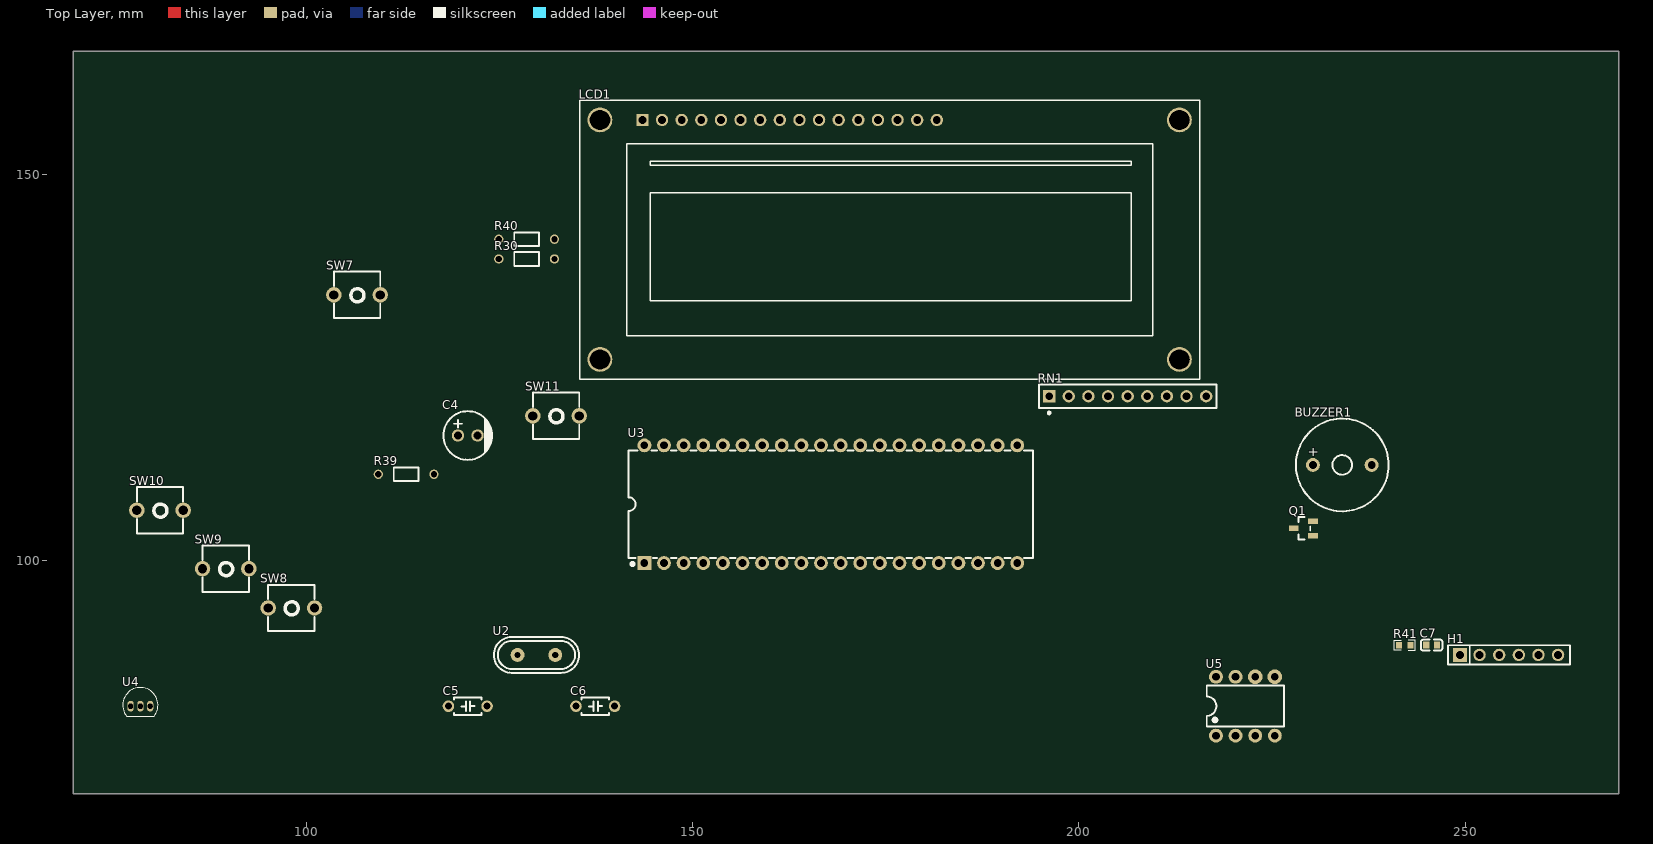
[diagram p0: Top Layer view]
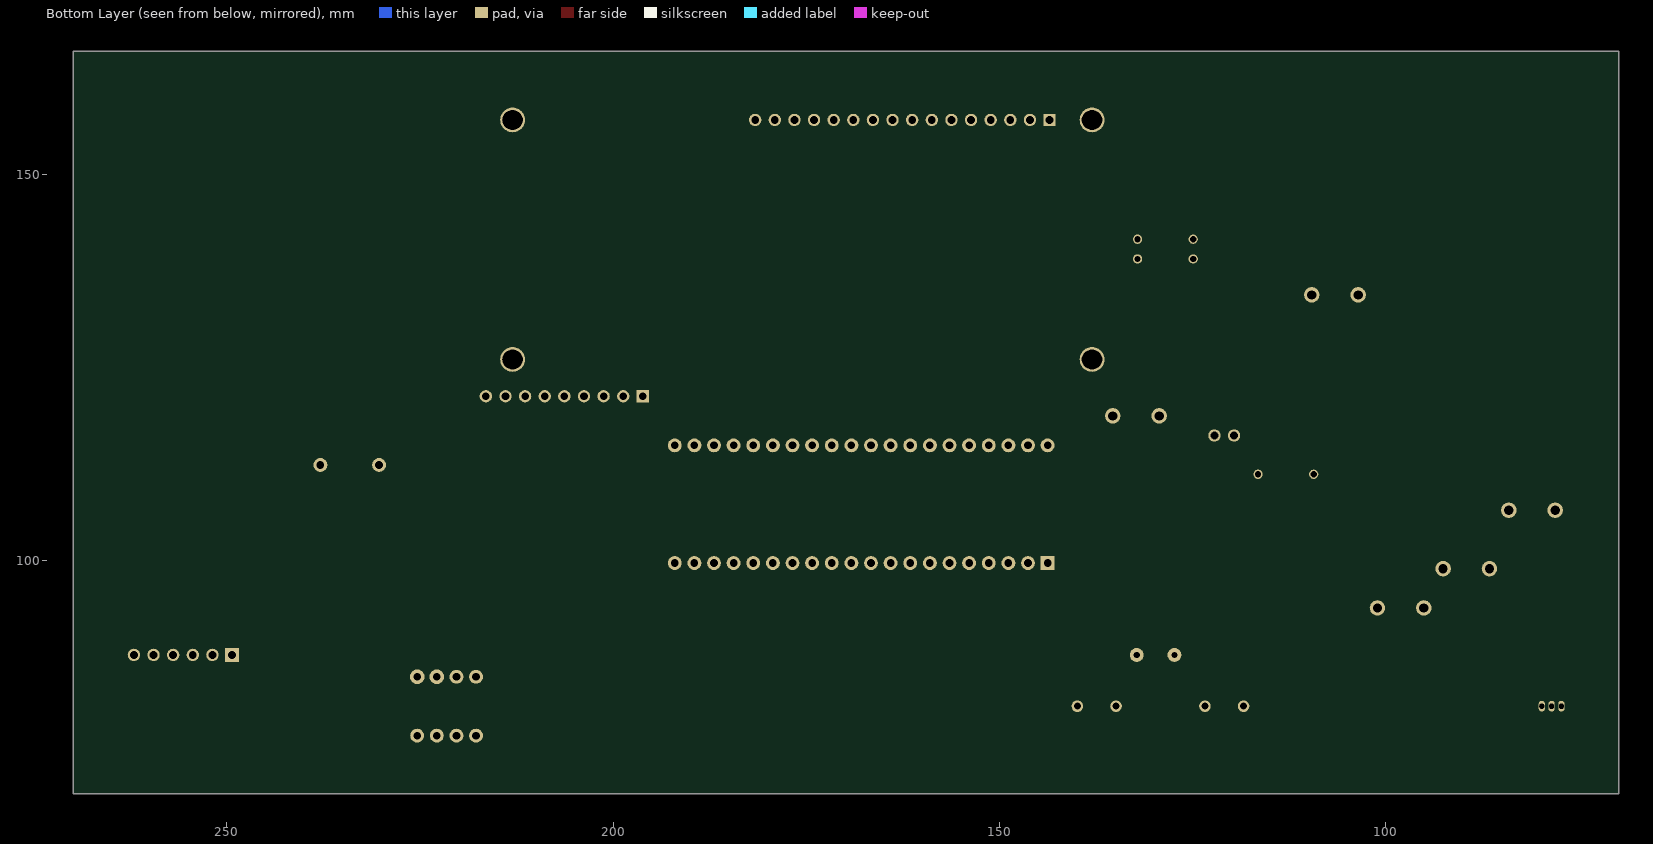
[diagram p1: Bottom Layer view, seen from below]
# Altium PCB MISC49895.pcbdoc
Units mm, origin at the board's own origin, x right, y up, seen from the top; angles counter-clockwise.
Board outline 200.06 x 96.14 mm, 2 copper layers (Top Layer, Bottom Layer), stack 1.58 mm thick; 22 components, 27 nets, 119 pads, 0 vias.

## Layer stack, top to bottom
Top Solder Mask Layer: solder mask 0.01, Dk 3.3
Top Layer: signal copper 0.035
Dielectric1: surface 1.51, FR4, Dk 4.5
Bottom Layer: signal copper 0.035
Bottom Solder Mask Layer: solder mask 0.01, Dk 3.3

## Board outline
269.911,69.85 69.85,69.85 69.85,165.986 269.911,165.986

## Design rules (kind name [scope] priority, off if disabled: settings)
BoardOutlineClearance copperThickness2oz_1 [All] p2 off: genericclearance=0.203 ignorepadtopadclearanceinfootprint=FALSE except(0: Arc-SplitContinuation Track-SplitContinuation SMDPad-SplitContinuation THPad-SplitContinuation Via-SplitContinuation Fill-SplitContinuation Region-SplitContinuation Poly-SplitContinuation Text-SplitContinuation Hole-SplitContinuation; 0.152: Arc-CutoutEdge Track-CutoutEdge SMDPad-CutoutEdge THPad-CutoutEdge Via-CutoutEdge Text-CutoutEdge; 0.175: Hole-OutlineEdge Hole-CutoutEdge; 0.254: Poly-OutlineEdge Poly-CutoutEdge; 0.3: Arc-OutlineEdge Track-OutlineEdge SMDPad-OutlineEdge THPad-OutlineEdge Via-OutlineEdge Fill-OutlineEdge Region-OutlineEdge Text-OutlineEdge Fill-CutoutEdge Region-CutoutEdge)
BoardOutlineClearance Plane_innerPlane_1 [All] p4 off: genericclearance=0.102 ignorepadtopadclearanceinfootprint=FALSE except(0: Arc-SplitContinuation Track-SplitContinuation SMDPad-SplitContinuation THPad-SplitContinuation Via-SplitContinuation Fill-SplitContinuation Region-SplitContinuation Poly-SplitContinuation Text-SplitContinuation Hole-SplitContinuation; 0.152: Arc-CutoutEdge Track-CutoutEdge SMDPad-CutoutEdge THPad-CutoutEdge Via-CutoutEdge Text-CutoutEdge; 0.175: Hole-OutlineEdge Hole-CutoutEdge; 0.254: Poly-OutlineEdge Poly-CutoutEdge; 0.3: Arc-OutlineEdge Track-OutlineEdge SMDPad-OutlineEdge THPad-OutlineEdge Via-OutlineEdge Fill-OutlineEdge Region-OutlineEdge Text-OutlineEdge Fill-CutoutEdge Region-CutoutEdge)
BoardOutlineClearance Copper_copperRegion_1 [All] p6 off: genericclearance=0.102 ignorepadtopadclearanceinfootprint=FALSE except(0: Arc-SplitContinuation Track-SplitContinuation SMDPad-SplitContinuation THPad-SplitContinuation Via-SplitContinuation Fill-SplitContinuation Region-SplitContinuation Poly-SplitContinuation Text-SplitContinuation Hole-SplitContinuation; 0.152: Arc-CutoutEdge Track-CutoutEdge SMDPad-CutoutEdge THPad-CutoutEdge Via-CutoutEdge Text-CutoutEdge; 0.175: Hole-OutlineEdge Hole-CutoutEdge; 0.254: Poly-OutlineEdge Poly-CutoutEdge; 0.3: Arc-OutlineEdge Track-OutlineEdge SMDPad-OutlineEdge THPad-OutlineEdge Via-OutlineEdge Fill-OutlineEdge Region-OutlineEdge Text-OutlineEdge Fill-CutoutEdge Region-CutoutEdge)
BoardOutlineClearance copperThickness1oz_1 [All] p8: genericclearance=0.102 ignorepadtopadclearanceinfootprint=FALSE except(0: Arc-SplitContinuation Track-SplitContinuation SMDPad-SplitContinuation THPad-SplitContinuation Via-SplitContinuation Fill-SplitContinuation Region-SplitContinuation Poly-SplitContinuation Text-SplitContinuation Hole-SplitContinuation; 0.152: Arc-CutoutEdge Track-CutoutEdge SMDPad-CutoutEdge THPad-CutoutEdge Via-CutoutEdge Text-CutoutEdge; 0.175: Hole-OutlineEdge Hole-CutoutEdge; 0.254: Poly-OutlineEdge Poly-CutoutEdge; 0.3: Arc-OutlineEdge Track-OutlineEdge SMDPad-OutlineEdge THPad-OutlineEdge Via-OutlineEdge Fill-OutlineEdge Region-OutlineEdge Text-OutlineEdge Fill-CutoutEdge Region-CutoutEdge)
Clearance copperThickness2oz [All] p1 off: gap=0.203 ignorepadtopadclearanceinfootprint=FALSE except(0.152: SMDPad-Track SMDPad-SMDPad THPad-Track SMDPad-THPad THPad-THPad Track-Via SMDPad-Via THPad-Via Via-Via Fill-SMDPad Region-SMDPad Fill-THPad Region-THPad Fill-Via Region-Via Fill-Fill Fill-Region Region-Region Arc-Track Arc-SMDPad Arc-THPad Arc-Via Fill-Arc Region-Arc Arc-Arc Text-Track SMDPad-Text Text-THPad Text-Via Fill-Text Region-Text Arc-Text Text-Text; 0.175: Hole-Track Hole-SMDPad Hole-THPad Hole-Via Fill-Hole Region-Hole Hole-Arc Hole-Text; 0.254: Poly-Track Poly-SMDPad Poly-THPad Poly-Via Poly-Fill Poly-Region Poly-Poly Poly-Arc Poly-Text Poly-Hole; 0.3: Fill-Track Region-Track)
Clearance Plane_innerPlane [All] p3 off: gap=0.102 ignorepadtopadclearanceinfootprint=FALSE except(0.152: SMDPad-Track SMDPad-SMDPad THPad-Track SMDPad-THPad THPad-THPad Track-Via SMDPad-Via THPad-Via Via-Via Fill-SMDPad Region-SMDPad Fill-THPad Region-THPad Fill-Via Region-Via Fill-Fill Fill-Region Region-Region Arc-Track Arc-SMDPad Arc-THPad Arc-Via Fill-Arc Region-Arc Arc-Arc Text-Track SMDPad-Text Text-THPad Text-Via Fill-Text Region-Text Arc-Text Text-Text; 0.175: Hole-Track Hole-SMDPad Hole-THPad Hole-Via Fill-Hole Region-Hole Hole-Arc Hole-Text; 0.254: Poly-Track Poly-SMDPad Poly-THPad Poly-Via Poly-Fill Poly-Region Poly-Poly Poly-Arc Poly-Text Poly-Hole; 0.3: Fill-Track Region-Track)
Clearance Copper_copperRegion [All] p5 off: gap=0.102 ignorepadtopadclearanceinfootprint=FALSE except(0.152: SMDPad-Track SMDPad-SMDPad THPad-Track SMDPad-THPad THPad-THPad Track-Via SMDPad-Via THPad-Via Via-Via Fill-SMDPad Region-SMDPad Fill-THPad Region-THPad Fill-Via Region-Via Fill-Fill Fill-Region Region-Region Arc-Track Arc-SMDPad Arc-THPad Arc-Via Fill-Arc Region-Arc Arc-Arc Text-Track SMDPad-Text Text-THPad Text-Via Fill-Text Region-Text Arc-Text Text-Text; 0.175: Hole-Track Hole-SMDPad Hole-THPad Hole-Via Fill-Hole Region-Hole Hole-Arc Hole-Text; 0.254: Poly-Track Poly-SMDPad Poly-THPad Poly-Via Poly-Fill Poly-Region Poly-Poly Poly-Arc Poly-Text Poly-Hole; 0.3: Fill-Track Region-Track)
Clearance copperThickness1oz [All] p7: gap=0.102 ignorepadtopadclearanceinfootprint=FALSE except(0.152: SMDPad-Track SMDPad-SMDPad THPad-Track SMDPad-THPad THPad-THPad Track-Via SMDPad-Via THPad-Via Via-Via Fill-SMDPad Region-SMDPad Fill-THPad Region-THPad Fill-Via Region-Via Fill-Fill Fill-Region Region-Region Arc-Track Arc-SMDPad Arc-THPad Arc-Via Fill-Arc Region-Arc Arc-Arc Text-Track SMDPad-Text Text-THPad Text-Via Fill-Text Region-Text Arc-Text Text-Text; 0.175: Hole-Track Hole-SMDPad Hole-THPad Hole-Via Fill-Hole Region-Hole Hole-Arc Hole-Text; 0.254: Poly-Track Poly-SMDPad Poly-THPad Poly-Via Poly-Fill Poly-Region Poly-Poly Poly-Arc Poly-Text Poly-Hole; 0.3: Fill-Track Region-Track)
DiffPairsRouting differentialPair [All] p1: maxlimit=0.152 minlimit=0.152 mostfreqgap=0.152 toplayer_minwidth=0.127 toplayer_prefwidth=0.254 toplayer_maxwidth=2.54 toplayer_mingap=0.152 toplayer_prefgap=0.152 toplayer_maxgap=0.152 bottomlayer_minwidth=0.127 bottomlayer_prefwidth=0.254 bottomlayer_maxwidth=2.54 bottomlayer_mingap=0.152 bottomlayer_prefgap=0.152 bottomlayer_maxgap=0.152 maxuncoupledlength=0.254
HoleToHoleClearance otherClearance [All] p1: gap=0.3 allowstackedmicrovias=TRUE
Length netLength [All] p1: minlimit=0 maxlimit=0
PasteMaskExpansion pasteMaskExpansion [All] p1: expansion=0
PlaneConnect innerPlane [All] p1: planeconnectstyle=Relief reliefexpansion=0.508 reliefentries=4 reliefconductorwidth=0.254 reliefairgap=0.254
PolygonConnect copperRegion [All] p1: connectstyle=Relief reliefconductorwidth=0.254 reliefentries=4 polygonreliefangle="90 Angle" airgapwidth=0.254 via.connectstyle=Relief via.reliefconductorwidth=0.254 via.reliefentries=4 via.polygonreliefangle="90 Angle" via.airgapwidth=0.254
RoutingVias viaSize [All] p1: holewidth=0.305 width=0.61 viastyle="Through Hole" minholewidth=0.3 minwidth=0.5 maxholewidth=6.3 maxwidth=10
SolderMaskExpansion solderMaskExpansion [IsVia] p1: expansion=-25.4 istentingtop=TRUE
SolderMaskExpansion solderMaskExpansion [All] p2: expansion=0.051 istentingtop=FALSE
Width copperThickness2oz_2 [All] p1 off: maxlimit=2.54 minlimit=0.203 preferedwidth=0.254
Width copperThickness1oz_2 [All] p2: maxlimit=2.54 minlimit=0.127 preferedwidth=0.254

## Components (designator, comment, footprint, x,y, rotation, side; value= is the part's Value field where it differs from the comment)
BUZZER1 "buzzer-12X9" BUZ-TH_BD12.0-P7.60-D0.6-FD 234.111,112.425 r0 top
C4 "10uF" CAP-TH_BD6.3-P2.50-D1.0-FD 120.925,116.235 r0 top
C5 "30pF" CAP-TH_L3.6-W2.3-P5.00-D0.5 120.925,81.199 r0 top
C6 "30pF" CAP-TH_L3.6-W2.3-P5.00-D0.5 137.435,81.199 r0 top
C7 "22pF" C0603 245.677,89.108 r0 top
H1 "" HDR-TH_6P-P2.54-V-F 255.691,87.838 r0 top
LCD1 "LMB162ADC" LCD1602 175.535,141.576 r0 top
Q1 "" S8550P_SOT 229.031,104.211 r0 top
R30 "1kΩ" Res_1/8W 128.545,139.024 r0 top
R39 "10kΩ" Res_1/8W 112.95,111.155 r0 top
R40 "10kΩ" Res_1/8W 128.545,141.576 r0 top
R41 "51K" R0603 242.199,89.108 r0 top
RN1 "-" RES-ARRAY-TH_9P-P2.54-D1.0 206.331,121.315 r0 top
SW7 "Tact switch, 6*6*5 plastic head, 260G, travel 0.25mm, through-hole, middle 2 pins" KEY-TH_2P-L6.0-W6.0-P5.00 106.6,134.433 r0 top
SW8 "Tact switch, 6*6*5 plastic head, 260G, travel 0.25mm, through-hole, middle 2 pins" KEY-TH_2P-L6.0-W6.0-P5.00 98.1,93.916 r0 top
SW9 "Tact switch, 6*6*5 plastic head, 260G, travel 0.25mm, through-hole, middle 2 pins" KEY-TH_2P-L6.0-W6.0-P5.00 89.6,98.996 r0 top
SW10 "Tact switch, 6*6*5 plastic head, 260G, travel 0.25mm, through-hole, middle 2 pins" KEY-TH_2P-L6.0-W6.0-P5.00 81.1,106.565 r0 top
SW11 "Tact switch, 6*6*5 plastic head, 260G, travel 0.25mm, through-hole, middle 2 pins" KEY-TH_2P-L6.0-W6.0-P5.00 132.355,118.775 r0 top
U2 "12MHz" HC-49US_L11.0-W4.6-P4.88 129.815,87.838 r0 top
U3 "STC89C516RD+40I-PDIP40" DIP-40_L52.3-W13.9-P2.54-LS15.2-BL 167.915,107.345 r0 top
U4 "DS18B20" TO-92-3_L4.6-W3.6-P1.27-L-1 78.56,81.199 r0 top
U5 "ADC0832BCN" PDIP-8_L9.6-W6.4-P2.54-LS7.6-BL 221.571,81.199 r0 top

## Footprints (in the part's own frame and the unit in brackets; to place one, negate y for a bottom-side part, rotate by r counter-clockwise, add the part's x,y. Pads: shape width x height; smd on the part's side, far side on the other; paste and mask are expansions set on the pad)
BUZ-TH_BD12.0-P7.60-D0.6-FD [mm]
  round 1.8 hole 1: 1(-3.8,0) 2(3.8,0)
  silkscreen extent -6,-6 6,6
C0603 [mm]
  rect 0.8x0.9 smd: 1(-0.7,0) 2(0.7,0)
  silkscreen extent -1.39,-0.71 1.39,0.71
CAP-TH_BD6.3-P2.50-D1.0-FD [mm]
  round 1.6 hole 1: 1(-1.27,0) 2(1.27,0)
  silkscreen extent -3.15,-3.15 3.17,3.15
CAP-TH_L3.6-W2.3-P5.00-D0.5 [mm]
  round 1.5 hole 0.9: 1(-2.5,0) 2(2.5,0)
  silkscreen extent -1.8,-1.15 1.8,1.15
DIP-40_L52.3-W13.9-P2.54-LS15.2-BL [mm]
  rect 1.8x1.8 hole 1: 1(-24.13,-7.62)
  round 1.8 hole 1: 2(-21.59,-7.62) 3(-19.05,-7.62) 4(-16.51,-7.62) 5(-13.97,-7.62) 6(-11.43,-7.62) 7(-8.89,-7.62) 8(-6.35,-7.62) 9(-3.81,-7.62) 10(-1.27,-7.62) 11(1.27,-7.62) 12(3.81,-7.62) 13(6.35,-7.62) 14(8.89,-7.62) 15(11.43,-7.62) 16(13.97,-7.62) 17(16.51,-7.62) 18(19.05,-7.62) 19(21.59,-7.62) 20(24.13,-7.62) 21(24.13,7.62) 22(21.59,7.62) 23(19.05,7.62) 24(16.51,7.62) 25(13.97,7.62) 26(11.43,7.62) 27(8.89,7.62) 28(6.35,7.62) 29(3.81,7.62) 30(1.27,7.62) 31(-1.27,7.62) 32(-3.81,7.62) 33(-6.35,7.62) 34(-8.89,7.62) 35(-11.43,7.62) 36(-13.97,7.62) 37(-16.51,7.62) 38(-19.05,7.62) 39(-21.59,7.62) 40(-24.13,7.62)
  silkscreen extent -26.16,-7.95 26.16,6.93
HC-49US_L11.0-W4.6-P4.88 [mm]
  round 1.8 hole 0.8: 1(-2.44,0) 2(2.44,0)
  silkscreen extent -5.51,-2.32 5.51,2.32
HDR-TH_6P-P2.54-V-F [mm]
  rect 1.8x1.8 hole 1.02: 1(-6.35,0)
  round 1.6 hole 1.02: 2(-3.81,0) 3(-1.27,0) 4(1.27,0) 5(3.81,0) 6(6.35,0)
  silkscreen extent -7.87,-1.25 7.87,1.25
KEY-TH_2P-L6.0-W6.0-P5.00 [mm]
  round 2 hole 1.2: 1(-3,0) 2(3,0)
  silkscreen extent -3,-3 3,3
LCD1602 [mm]
  round 3.2 hole 2.5 slot 2.625 at 0 deg: 0(-37.5,-15.5) 0(-37.5,15.5) 0(37.5,-15.5) 0(37.5,15.5)
  rect 1.6x1.6 hole 1: 1(-32,15.5)
  round 1.6 hole 1: 2(-29.46,15.5) 3(-26.92,15.5) 4(-24.38,15.5) 5(-21.84,15.5) 6(-19.3,15.5) 7(-16.76,15.5) 8(-14.22,15.5) 9(-11.68,15.5) 10(-9.14,15.5) 11(-6.6,15.5) 12(-4.06,15.5) 13(-1.52,15.5) 14(1.02,15.5) 15(3.56,15.5) 16(6.1,15.5)
  silkscreen extent -40.13,-18.03 40.13,18.03
PDIP-8_L9.6-W6.4-P2.54-LS7.6-BL [mm]
  round 1.8 hole 1: 1(-3.81,-3.81) 2(-1.27,-3.81) 3(1.27,-3.81) 4(3.81,-3.81) 7(-1.27,3.81) 8(-3.81,3.81)
  round 1.905 hole 1: 5(3.81,3.81) 6(1.27,3.81)
  silkscreen extent -5,-2.64 5,2.67
R0603 [mm]
  rect 0.806x0.864 smd paste-100 mask+0.051: 1(-0.753,0) 2(0.753,0)
  silkscreen extent -1.39,-0.66 1.39,0.66
RES-ARRAY-TH_9P-P2.54-D1.0 [mm]
  rect 1.6x1.6 hole 1: 1(-10.16,0)
  round 1.6 hole 1: 2(-7.62,0) 3(-5.08,0) 4(-2.54,0) 5(0,0) 6(2.54,0) 7(5.08,0) 8(7.62,0) 9(10.16,0)
  silkscreen extent -11.5,-2.31 11.5,1.5
Res_1/8W [mil]
  round 47.2 hole 31.5 paste+0 mask+2: 1(-141.7,2.48) 2(141.7,2.48)
  silkscreen extent -63,-33 63,38
S8550P_SOT [mm]
  rect 1.25x0.701 smd paste+0 mask+0.051: 1(1.291,-0.95) 2(1.291,0.95) 3(-1.208,0)
  silkscreen extent -0.61,-1.46 0.94,1.46
TO-92-3_L4.6-W3.6-P1.27-L-1 [mm]
  oval 0.8x1.4 hole 0.6 slot 0.682 at 90 deg paste+0 mask+0.05: 1(-1.27,0) 2(0,0) 3(1.27,0)
  silkscreen extent -2.28,-1.28 2.28,2.41

## Nets (pads, with @x,y where several pads share a name; then routed paths per layer and width w, separated by ;. In a path a pad name is that pad's centre, name@x,y a point inside that pad or via, vN(x,y) a via of type N, cw(c..) or ccw(c..) an arc to the next point about the centre after c; other vN are vias at no path point)
$1N1586: LCD1.14 RN1.9 U3.32
$1N1590: LCD1.7 RN1.2 U3.39
$1N1591: LCD1.8 RN1.3 U3.38
$1N1592: LCD1.9 RN1.4 U3.37
$1N1593: LCD1.10 RN1.5 U3.36
$1N1594: LCD1.11 RN1.6 U3.35
$1N1595: LCD1.12 RN1.7 U3.34
$1N1596: LCD1.13 RN1.8 U3.33
$1N1605: LCD1.3 R30.2 R40.1
$1N1611: C5.2 U2.1 U3.18
$1N1612: C6.2 U2.2 U3.19
$1N1662: C4.2 R39.2 SW11.2 U3.9
$1N19376: SW7.2 U3.8
$1N19435: SW10.2 U3.10
$1N19444: SW9.2 U3.11
$1N19454: SW8.2 U3.12
$1N19651: U3.17 U4.2
$1N19796: U3.23 U5.1
$1N19863: U3.24 U5.7
$1N19872: U3.25 U5.5 U5.6
$1N19973: C7.2 H1.1 R41.2 U5.2
$1N20248: BUZZER1.2 Q1.2
EN: LCD1.6
GND: C5.1 C6.1 C7.1 H1.2 LCD1.1 LCD1.16 Q1.3 R30.1 R39.1 R41.1 SW7.1 SW8.1 SW9.1 SW10.1 U3.20 U4.1 U5.4
RS: LCD1.4
RW: LCD1.5
VCC: BUZZER1.1 C4.1 H1.3 LCD1.2 LCD1.15 R40.2 RN1.1 SW11.1 U3.40 U4.3 U5.8
pads on no net: H1.4 H1.5 H1.6 LCD1.0 Q1.1 U3.1 U3.2 U3.3 U3.4 U3.5 U3.6 U3.7 U3.13 U3.14 U3.15 U3.16 U3.21 U3.22 U3.26 U3.27 U3.28 U3.29 U3.30 U3.31 U5.3